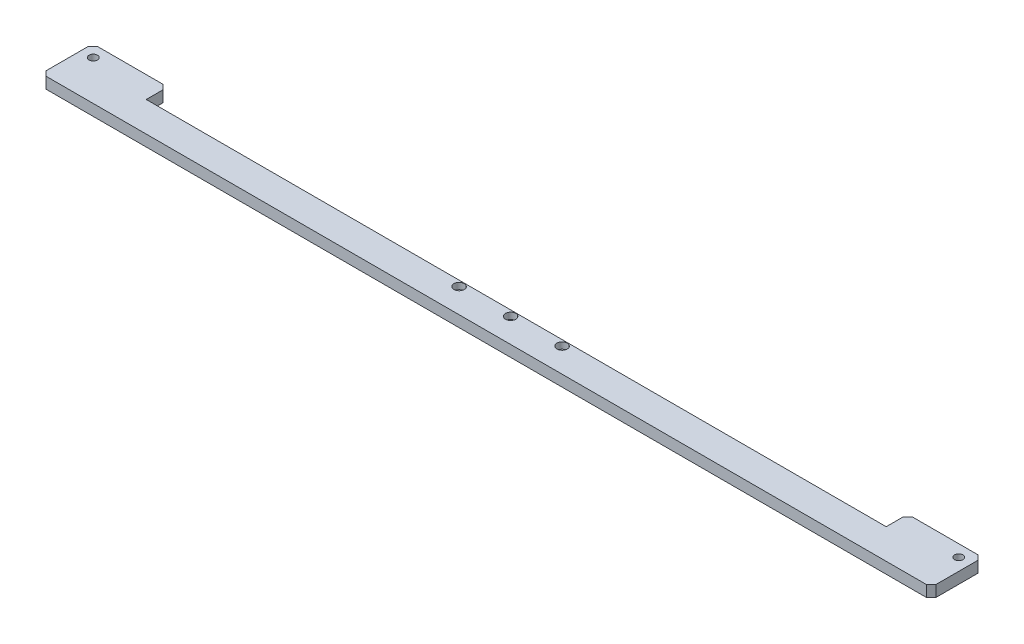
from build123d import *

# Parameters (mm, degrees)
SKETCH_1_W                = 950
SKETCH_1_H                = 55
EXTRUDE_1_DEPTH           = 6
SKETCH_2_W                = 790
SKETCH_2_H                = 23
CUT_EXTRUDE_1_DEPTH       = 12
CHAMFER_1_SIZE            = 5
HOLE_WIZARD_M8_1_D        = 9
HOLE_WIZARD_1_D           = 6.6
HOLE_WIZARD_1_CBORE_D     = 11
HOLE_WIZARD_1_CBORE_DEPTH = 6.8


with BuildPart() as part:
    # 草图1 → 凸台-拉伸1 (new, symmetric)
    with BuildSketch(Plane(origin=(0, 0, 0), x_dir=(1, 0, 0), z_dir=(0, 1, 0))):
        Rectangle(SKETCH_1_W, SKETCH_1_H)
    extrude(amount=EXTRUDE_1_DEPTH, both=True)

    # 草图2 → 切除-拉伸1 (cut)
    with BuildSketch(Plane(origin=(0, 6, 0), x_dir=(1, 0, 0), z_dir=(0, 1, 0))):
        with Locations((0, 16)):
            Rectangle(SKETCH_2_W, SKETCH_2_H)
    extrude(amount=-CUT_EXTRUDE_1_DEPTH, mode=Mode.SUBTRACT)

    # 倒角1
    chamfer_1_edges = [part.edges().sort_by_distance(p)[0] for p in [
        (-395, 0, -27.5),
        (395, 0, -27.5),
        (475, 0, 27.5),
        (-475, 0, 27.5),
        (-475, 0, -27.5),
        (475, 0, -27.5),
    ]]
    chamfer(chamfer_1_edges, length=CHAMFER_1_SIZE)

    # M8 间隙孔1 (through all)
    with Locations(Plane(origin=(0, -6, 0), x_dir=(-1, 0, 0), z_dir=(0, -1, 0))):
        with Locations((462, 15), (-462, 15)):
            Hole(HOLE_WIZARD_M8_1_D / 2)

    # 打孔尺寸(%根据)内六角圆柱头螺钉的类型1 (through all)
    with Locations(Plane(origin=(0, 6, 0), x_dir=(1, 0, 0), z_dir=(0, 1, 0))):
        with Locations((55, -1.5), (0, -1.5), (-55, -1.5)):
            CounterBoreHole(HOLE_WIZARD_1_D / 2, HOLE_WIZARD_1_CBORE_D / 2, HOLE_WIZARD_1_CBORE_DEPTH)


solid = part.part
